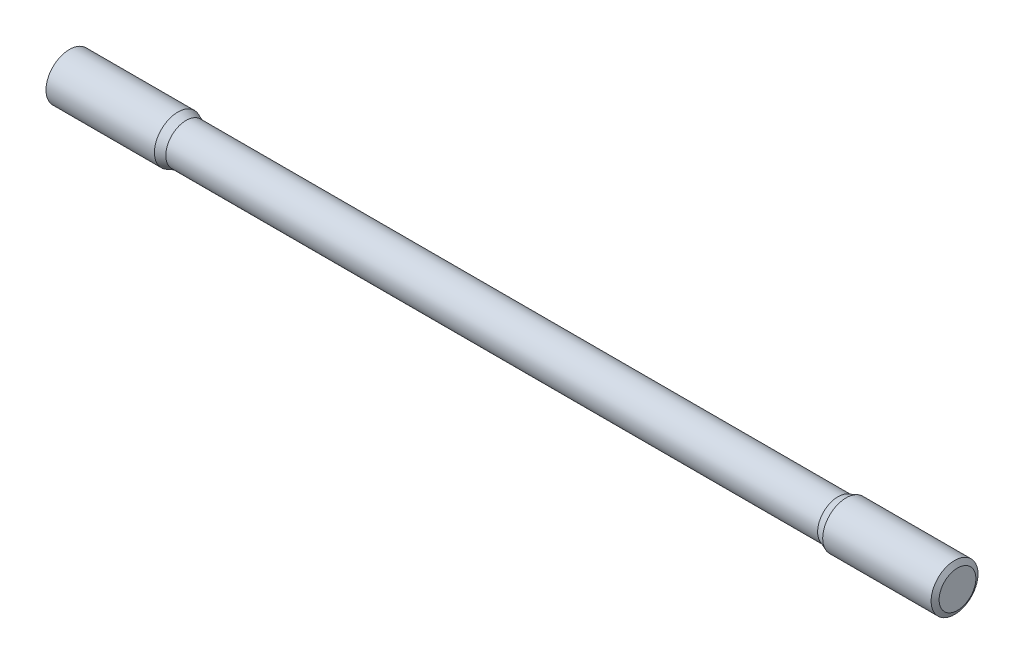
from build123d import *


with BuildPart() as part:
    # 草图1 → Revolve 558 (revolve)
    with BuildSketch(Plane.XY, mode=Mode.PRIVATE) as revolve_558_sk:
        Polygon((-152, 8), (-114, 8), (-111.2, 6.928), (111.2, 6.928), (114, 8), (152, 8), (152, 0), (-152, 0), align=None)
    revolve(revolve_558_sk.sketch.rotate(Axis((-152, 0, 0), (1, 0, 0)), 180), axis=Axis((-152, 0, 0), (1, 0, 0)))

    # 草图2 → Cut-Revolve 607 (revolve, cut)
    with BuildSketch(Plane.XY, mode=Mode.PRIVATE) as cut_revolve_607_sk:
        Polygon((-152.999970666, 8), (-151.000029334, 8), (-152, 6.268), align=None)
    cut_revolve_607 = revolve(cut_revolve_607_sk.sketch.rotate(Axis((-26.952426469, 0, 0), (1, 0, 0)), 180), axis=Axis((-26.952426469, 0, 0), (1, 0, 0)), mode=Mode.SUBTRACT)

    # 镜向1: Cut-Revolve 607 across plane
    add(cut_revolve_607.mirror(Plane(origin=(0, 0, 0), x_dir=(0, 0, 1), z_dir=(1, 0, 0))), mode=Mode.SUBTRACT)


solid = part.part
